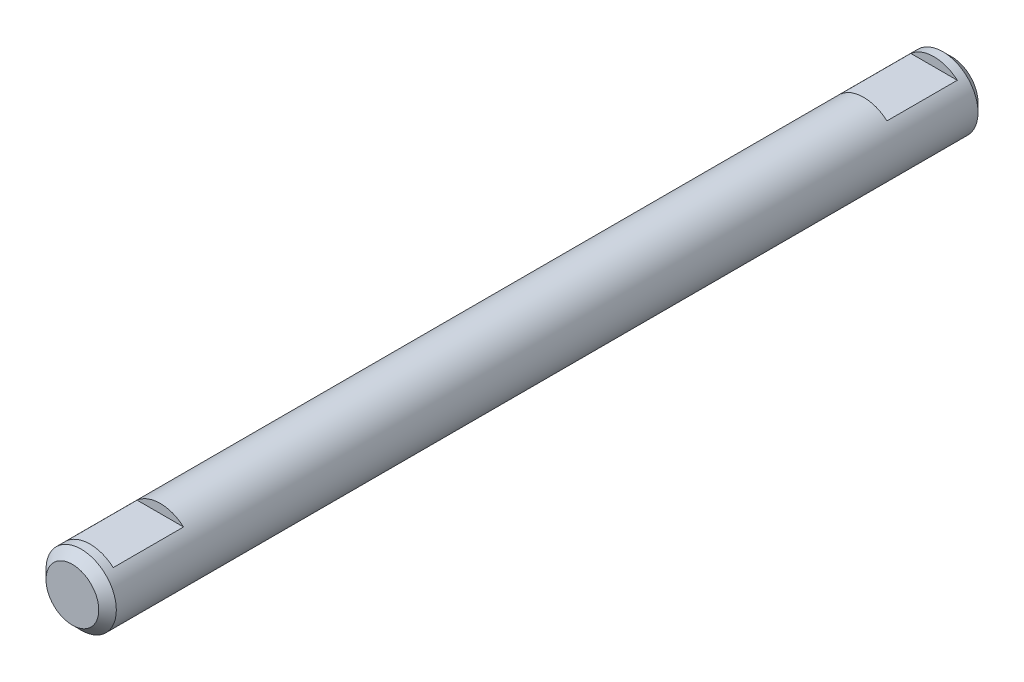
from build123d import *

# Parameters (mm, degrees)
SKETCH1_R           = 2
BOSS_EXTRUDE1_DEPTH = 25
SKETCH2_W           = 15.41853157
SKETCH2_H           = 4
SKETCH2_W_2         = 11.817796653
CUT_EXTRUDE1_DEPTH  = 0.5
CHAMFER1_SIZE       = 0.5


with BuildPart() as part:
    # Sketch1 → Boss-Extrude1 (new, symmetric)
    with BuildSketch(Plane.XY):
        Circle(SKETCH1_R)
    extrude(amount=BOSS_EXTRUDE1_DEPTH, both=True)

    # Sketch2 → Cut-Extrude1 (cut)
    with BuildSketch(Plane(origin=(0, 2, 0), x_dir=(-1, 0, 0), z_dir=(0, 1, 0))):
        with Locations((0, 22)):
            Rectangle(SKETCH2_W, SKETCH2_H)
        with Locations((0.877102096, -22)):
            Rectangle(SKETCH2_W_2, SKETCH2_H)
    extrude(amount=-CUT_EXTRUDE1_DEPTH, mode=Mode.SUBTRACT)

    # Chamfer1
    chamfer1_edges = [part.edges().sort_by_distance(p)[0] for p in [
        (-2, 0, -25),
        (-2, 0, 25),
    ]]
    chamfer(chamfer1_edges, length=CHAMFER1_SIZE)


solid = part.part
